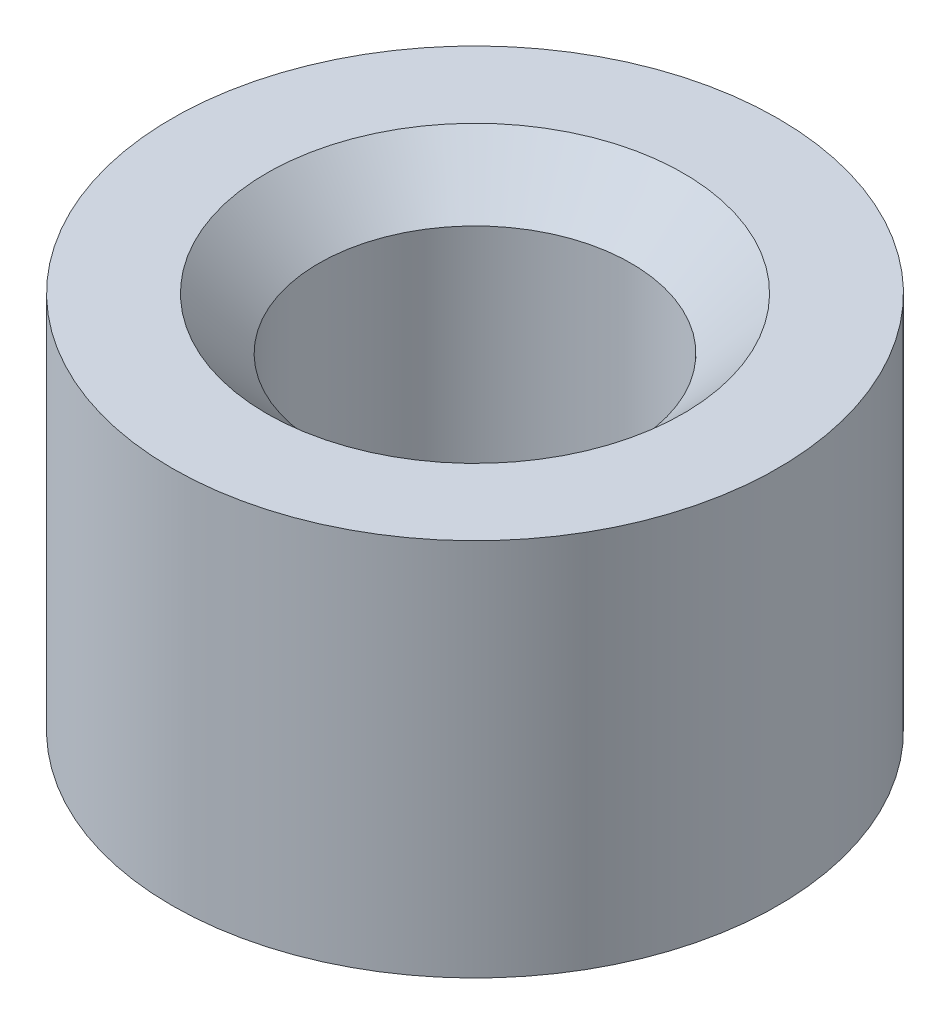
from build123d import *

# Parameters (mm, degrees)
SKETCH1_R                  = 16
SKETCH1_R_2                = 7.5
BOSS_EXTRUDE1_DEPTH        = 20
M18X1_5_TAPPED_HOLE2_D     = 16.5
M18X1_5_TAPPED_HOLE2_DEPTH = 30
M18X1_5_TAPPED_HOLE2_TIP   = 4.957100107
CHAMFER1_SIZE              = 2.75


with BuildPart() as part:
    # Sketch1 → Boss-Extrude1 (new body)
    with BuildSketch(Plane(origin=(0, 0, 0), x_dir=(1, 0, 0), z_dir=(0, 1, 0))):
        with Locations(Location((0, 0, 0), (0, 0, 270))):
            Circle(SKETCH1_R)
        with Locations(Location((0, 0, 0), (0, 0, 270))):
            Circle(SKETCH1_R_2, mode=Mode.SUBTRACT)
    extrude(amount=BOSS_EXTRUDE1_DEPTH)

    # M18x1.5 Tapped Hole2
    with Locations(Plane(origin=(0, 20, 0), x_dir=(1, 0, 0), z_dir=(0, 1, 0))):
        with Locations((0, 0)):
            Hole(M18X1_5_TAPPED_HOLE2_D / 2, depth=M18X1_5_TAPPED_HOLE2_DEPTH)
            with Locations((0, 0, -(M18X1_5_TAPPED_HOLE2_DEPTH + M18X1_5_TAPPED_HOLE2_TIP / 2))):  # 118° drill point
                Cone(0, M18X1_5_TAPPED_HOLE2_D / 2, M18X1_5_TAPPED_HOLE2_TIP, mode=Mode.SUBTRACT)

    # Chamfer1
    chamfer1_edges = [part.edges().sort_by_distance(p)[0] for p in [
        (8.25, 20, 0),
    ]]
    chamfer(chamfer1_edges, length=CHAMFER1_SIZE)


solid = part.part
